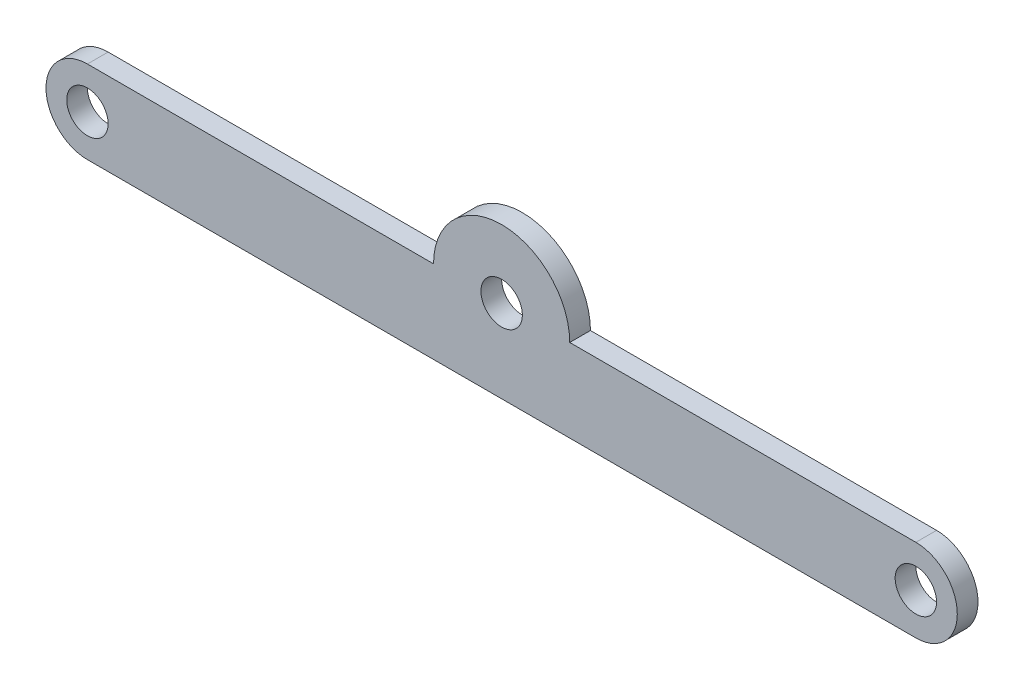
SolidWorks part; units mm, degrees
ref_plane "Front Plane" through (0, 0, 0) normal (0, 0, 1) x (1, 0, 0)
ref_plane "Top Plane" through (0, 0, 0) normal (0, 1, 0) x (1, 0, 0)
ref_plane "Right Plane" through (0, 0, 0) normal (1, 0, 0) x (0, 0, -1)
sketch "Sketch1" plane through (0, 0, 0) normal (0, 0, 1) x (1, 0, 0)
  line L0 (-200, 0) -> (200, 0) construction
  line L1 (-200, 20) -> (200, 20)
  line L2 (-200, -20) -> (200, -20)
  arc A0 (-200, 20) -> (-200, -20) centre (-200, 0) ccw
  arc A1 (200, -20) -> (200, 20) centre (200, 0) ccw
  point P2 (0, 0)
  dimension "D1" = 20
  dimension "D2" = 400
extrude "Boss-Extrude1" add sketch "Sketch1" along normal blind 10
sketch "Sketch2" plane through (0, 0, 10) normal (0, 0, 1) x (1, 0, 0)
  circle A0 centre (-200, 0) radius 10
  circle A1 centre (200, 0) radius 10
  dimension "D1" = 20
extrude "Cut-Extrude1" cut sketch "Sketch2" against normal through all
sketch "Sketch4" plane through (0, 0, 10) normal (0, 0, 1) x (1, 0, 0)
  line L0 (200, 20) -> (-200, 20) construction
  circle A0 centre (0, 20) radius 32.8789
extrude "Boss-Extrude2" add sketch "Sketch4" against normal up to surface (10 mm away) up to face at (-190, 0, 0)
sketch "Sketch5" plane through (0, 0, 10) normal (0, 0, 1) x (1, 0, 0)
  circle A0 centre (0, 20) radius 10
  dimension "D1" = 20
extrude "Cut-Extrude3" cut sketch "Sketch5" against normal through all
